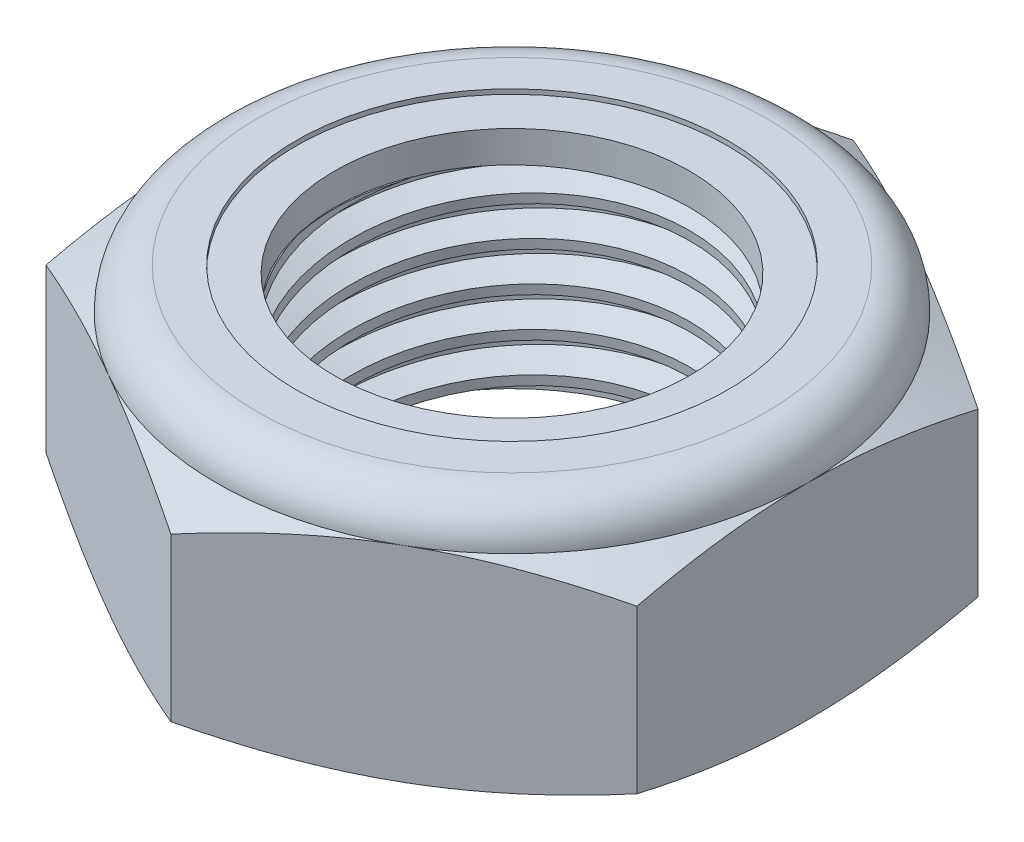
from build123d import *

# Parameters (mm, degrees)
EXTRUDE1_DEPTH      = 7.9375
SKETCH2_W           = 6.35
SKETCH2_H           = 7.9375
LPATTERN1_COUNT     = 6
LPATTERN1_PITCH     = 1.27
LPATTERN1_COL_COUNT = 2
LPATTERN1_COL_PITCH = 1.27


with BuildPart() as part:
    # Sketch1 → Extrude1 (new body)
    with BuildSketch(Plane(origin=(0, 0, 0), x_dir=(1, 0, 0), z_dir=(0, 1, 0))):
        Polygon((0, 10.998522628), (-9.525, 5.499261314), (-9.525, -5.499261314), (0, -10.998522628), (9.525, -5.499261314), (9.525, 5.499261314), align=None)
    extrude(amount=EXTRUDE1_DEPTH)

    # Sketch4 → Cut-Revolve2 (revolve, cut)
    with BuildSketch(Plane(origin=(0, 0, 0), x_dir=(0, 0, -1), z_dir=(1, 0, 0)), mode=Mode.PRIVATE) as cut_revolve2_sk:
        Polygon((0, 7.9375), (6.35, 7.9375), (5.721290563, 7.644327975), (5.721290563, 0.293172025), (6.35, 0), (0, 0), align=None)
    revolve(cut_revolve2_sk.sketch.rotate(Axis((0, 7.9375, 0), (0, 1, 0)), 54.6652943), axis=Axis((0, 7.9375, 0), (0, 1, 0)), mode=Mode.SUBTRACT)


with BuildPart() as body_2:
    # Sketch2 → Revolve1 (revolve)
    with BuildSketch(Plane(origin=(0, 0, 0), x_dir=(0, 0, -1), z_dir=(1, 0, 0))):
        with Locations((3.175, 3.96875)):
            Rectangle(SKETCH2_W, SKETCH2_H)
    revolve(axis=Axis((0, -6.35, 0), (0, 1, 0)))

    # Sketch3 → Cut-Revolve1 (revolve, cut)
    with BuildSketch(Plane(origin=(0, 0, 0), x_dir=(0, 0, -1), z_dir=(1, 0, 0)), mode=Mode.PRIVATE) as cut_revolve1_sk:
        Polygon((6.365796215, 7.779537846), (6.476369723, 6.673802768), (5.752882994, 7.000308534), (5.721290563, 7.316232842), align=None)
    cut_revolve1 = revolve(cut_revolve1_sk.sketch.rotate(Axis((0, 7.9375, 0.135293799), (0, -0.9950371902099892, -0.09950371902099908)), 180), axis=Axis((0, 7.9375, 0.135293799), (0, -0.9950371902099892, -0.09950371902099908)), mode=Mode.SUBTRACT)

    # LPattern1: Cut-Revolve1 ×6
    with Locations(*[(0, -i * LPATTERN1_PITCH, 0) for i in range(1, LPATTERN1_COUNT)]):
        add(cut_revolve1, mode=Mode.SUBTRACT)

    # LPattern1 col: Cut-Revolve1 ×2
    with Locations(*[(0, i * LPATTERN1_COL_PITCH, 0) for i in range(1, LPATTERN1_COL_COUNT)]):
        add(cut_revolve1, mode=Mode.SUBTRACT)


with BuildPart() as part_1:
    add(part.part)

    # Combine1: cut body 2
    add(body_2.part, mode=Mode.SUBTRACT)

    # Sketch5 → Cut-Revolve3 (revolve, cut)
    with BuildSketch(Plane(origin=(0, 0, 0), x_dir=(0, 0, -1), z_dir=(1, 0, 0)), mode=Mode.PRIVATE) as cut_revolve3_sk:
        with BuildLine():
            Line((0, 0), (9.525, 0))
            Line((9.525, 0), (10.998522628, 0.687114886))
            Line((10.998522628, 0.687114886), (10.998522628, 5.927468447))
            Line((10.998522628, 5.927468447), (9.525, 6.614583333))
            ThreePointArc((9.525, 6.614583333), (9.137526679, 7.550026679), (8.202083333, 7.9375))
            Line((8.202083333, 7.9375), (8.202083333, 9.2075))
            Line((8.202083333, 9.2075), (12.268522628, 9.2075))
            Line((12.268522628, 9.2075), (12.268522628, -1.27))
            Line((12.268522628, -1.27), (0, -1.27))
            Line((0, -1.27), (0, 0))
        make_face()
    revolve(cut_revolve3_sk.sketch.rotate(Axis((0, 0, 0), (0, 1, 0)), 54.6652943), axis=Axis((0, 0, 0), (0, 1, 0)), mode=Mode.SUBTRACT)

    # Sketch6 → Cut-Revolve4 (revolve, cut)
    with BuildSketch(Plane(origin=(0, 0, 0), x_dir=(0, 0, -1), z_dir=(1, 0, 0)), mode=Mode.PRIVATE) as cut_revolve4_sk:
        with BuildLine():
            Line((0, 6.614583333), (9.3726, 6.614583333))
            ThreePointArc((9.3726, 6.614583333), (9.029763606, 7.442263606), (8.202083333, 7.7851))
            Line((8.202083333, 7.7851), (6.961686948, 7.7851))
            Line((6.961686948, 7.7851), (6.961686948, 9.2075))
            Line((6.961686948, 9.2075), (0, 9.2075))
            Line((0, 9.2075), (0, 6.614583333))
        make_face()
    revolve(cut_revolve4_sk.sketch.rotate(Axis((0, 9.2075, 0), (0, 1, 0)), 54.6652943), axis=Axis((0, 9.2075, 0), (0, 1, 0)), mode=Mode.SUBTRACT)


with BuildPart() as body_2_2:
    # Sketch7 → Revolve2 (revolve)
    with BuildSketch(Plane(origin=(0, 0, 0), x_dir=(0, 0, -1), z_dir=(1, 0, 0))):
        with BuildLine():
            Line((5.721290563, 6.690783333), (9.293743778, 6.690783333))
            ThreePointArc((9.293743778, 6.690783333), (8.948455237, 7.4148695), (8.202083333, 7.7089))
            Line((8.202083333, 7.7089), (5.721290563, 7.7089))
            Line((5.721290563, 7.7089), (5.721290563, 6.690783333))
        make_face()
    revolve(axis=Axis((0, 6.690783333, 0), (0, 1, 0)))


solid = Compound([part_1.part, body_2_2.part])
